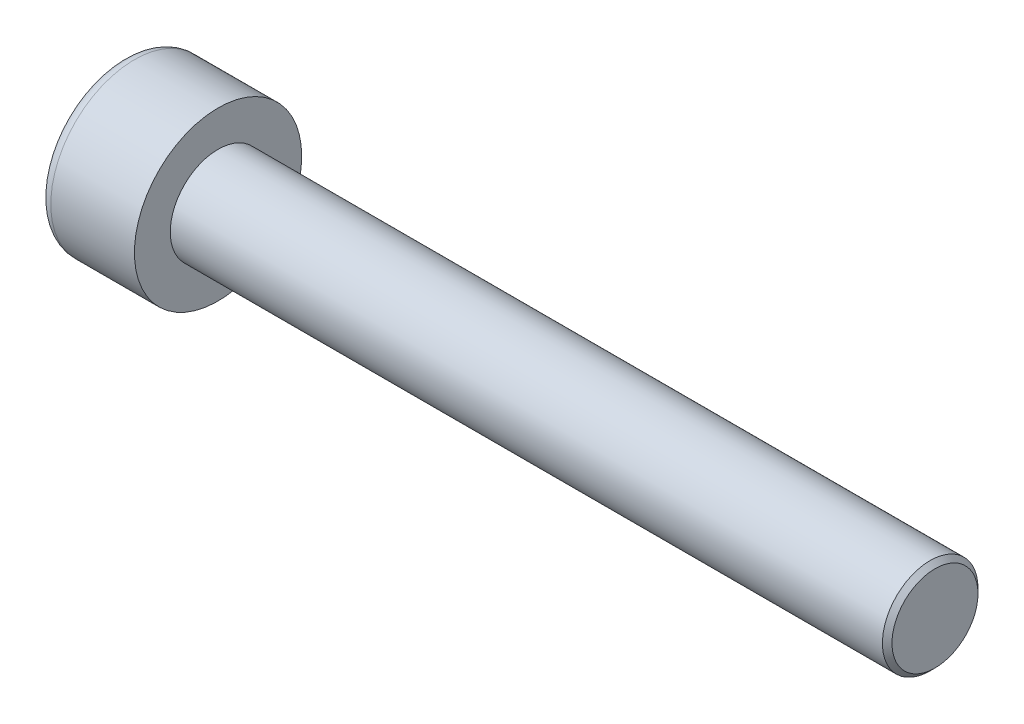
from build123d import *

# Parameters (mm, degrees)
SKETCH1_R           = 3.5
BASEHEAD_DEPTH      = 4
SKETCH2_R           = 2
BASEBODY_DEPTH      = 30
HEXAGONSOCKET_DEPTH = 2
TOPFILLET_R         = 0.5
CHAMFER1_SIZE       = 0.2


with BuildPart() as part:
    # Sketch1 → BaseHead (new body)
    with BuildSketch(Plane(origin=(0, 0, 0), x_dir=(0, 0, -1), z_dir=(1, 0, 0))):
        Circle(SKETCH1_R)
    extrude(amount=BASEHEAD_DEPTH)

    # Sketch2 → BaseBody (add)
    with BuildSketch(Plane(origin=(4, 0, 0), x_dir=(0, 0, -1), z_dir=(1, 0, 0))):
        Circle(SKETCH2_R)
    extrude(amount=BASEBODY_DEPTH)

    # Sketch3 → HexagonSocket (cut)
    with BuildSketch(Plane(origin=(0, 0, 0), x_dir=(0, 0, -1), z_dir=(1, 0, 0))):
        Polygon((1.732050808, 0), (0.866025404, 1.5), (-0.866025404, 1.5), (-1.732050808, 0), (-0.866025404, -1.5), (0.866025404, -1.5), align=None)
    extrude(amount=HEXAGONSOCKET_DEPTH, mode=Mode.SUBTRACT)

    # Sketch4 → Cut-Revolve1 (revolve, cut)
    with BuildSketch(Plane(origin=(-4.19613823, 0.75, 0), x_dir=(-1, 0, 0), z_dir=(0, 0, 1)), mode=Mode.PRIVATE) as cut_revolve1_sk:
        Polygon((-6.19613823, 2.25), (-7.062163633, 0.75), (-6.19613823, 0.75), align=None)
    revolve(cut_revolve1_sk.sketch.rotate(Axis((0.838992387, 0, 0), (-1, 0, 0)), 90), axis=Axis((0.838992387, 0, 0), (-1, 0, 0)), mode=Mode.SUBTRACT)

    # TopFillet
    topfillet_edges = [part.edges().sort_by_distance(p)[0] for p in [
        (0, 0, 3.5),
    ]]
    fillet(topfillet_edges, radius=TOPFILLET_R)

    # Chamfer1
    chamfer1_edges = [part.edges().sort_by_distance(p)[0] for p in [
        (34, 0, 2),
    ]]
    chamfer(chamfer1_edges, length=CHAMFER1_SIZE)


solid = part.part
